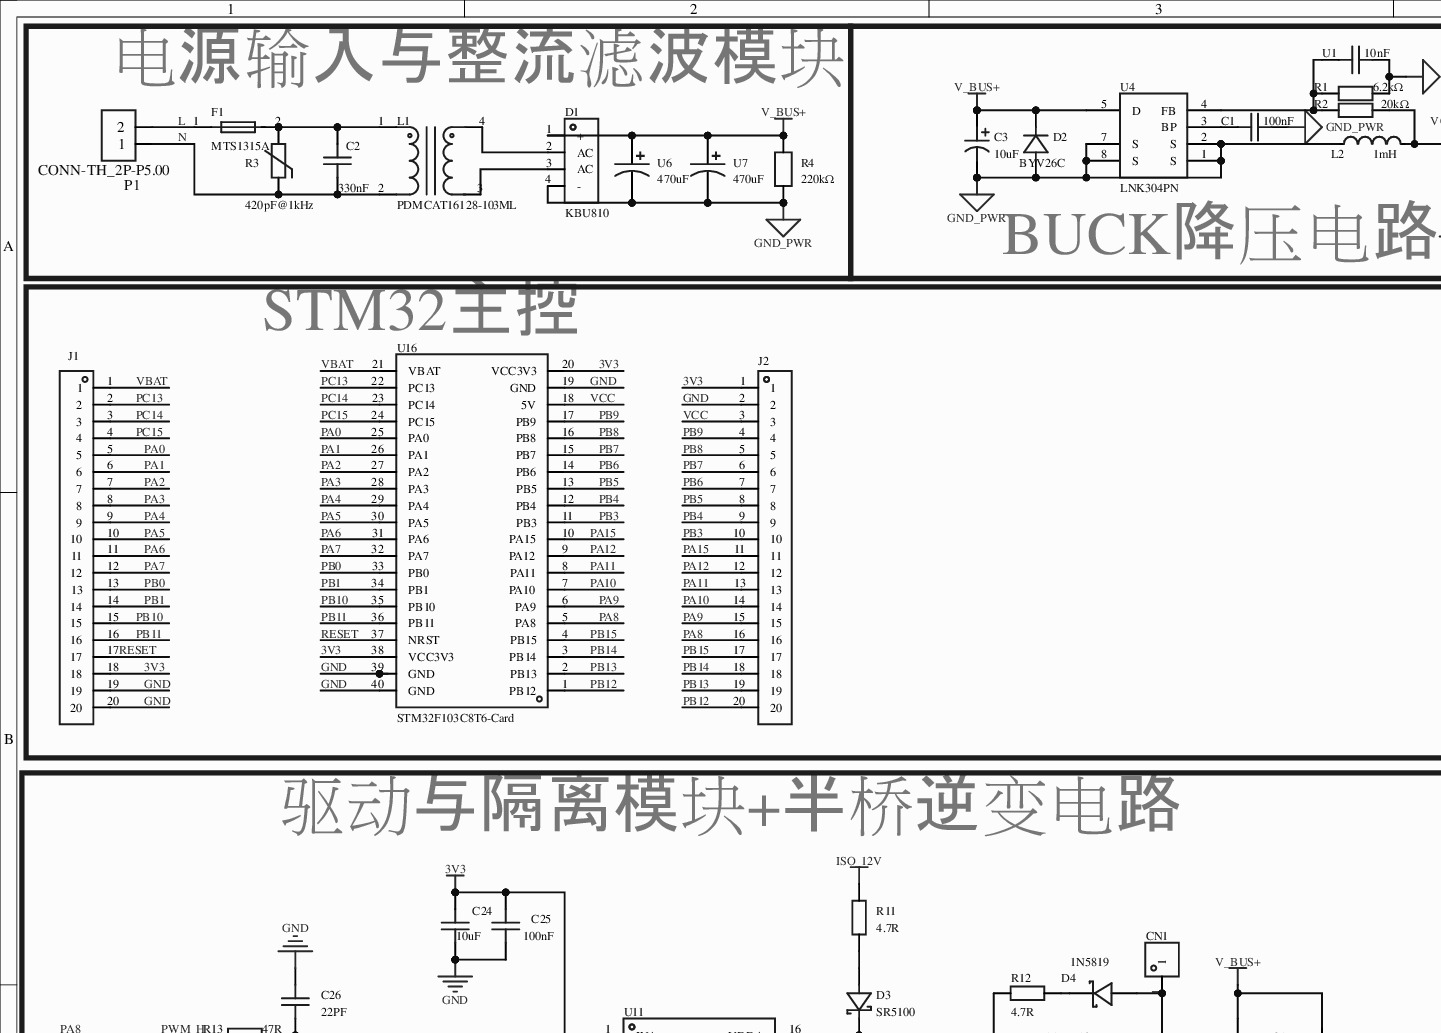
[diagram p0: MISC51807-3.schdoc, top left]
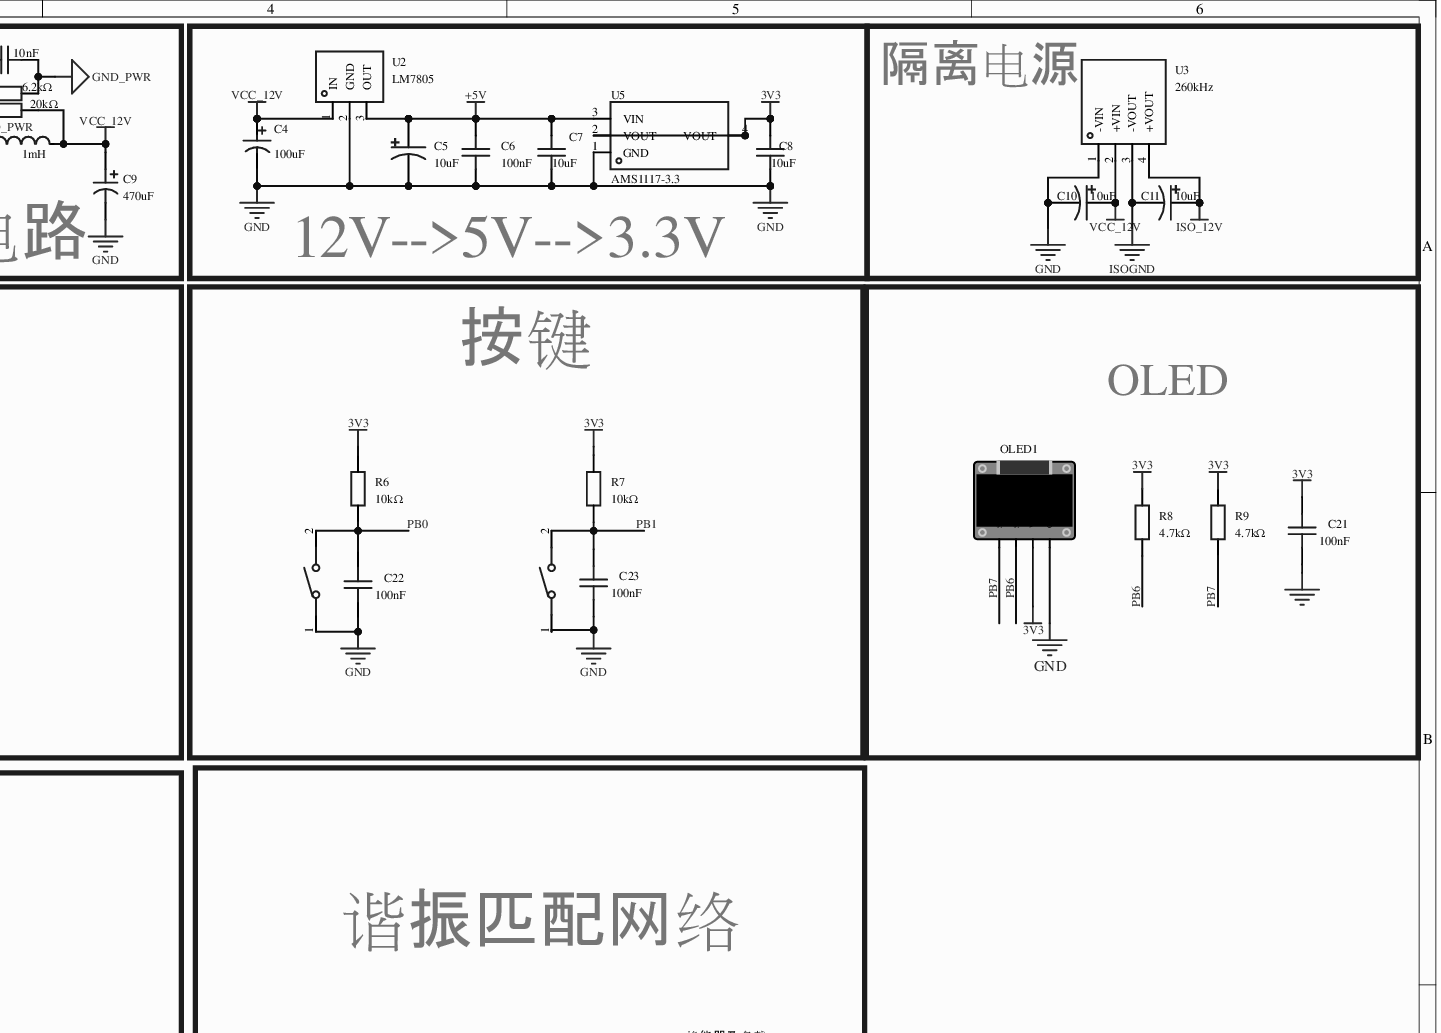
[diagram p1: MISC51807-3.schdoc, top right]
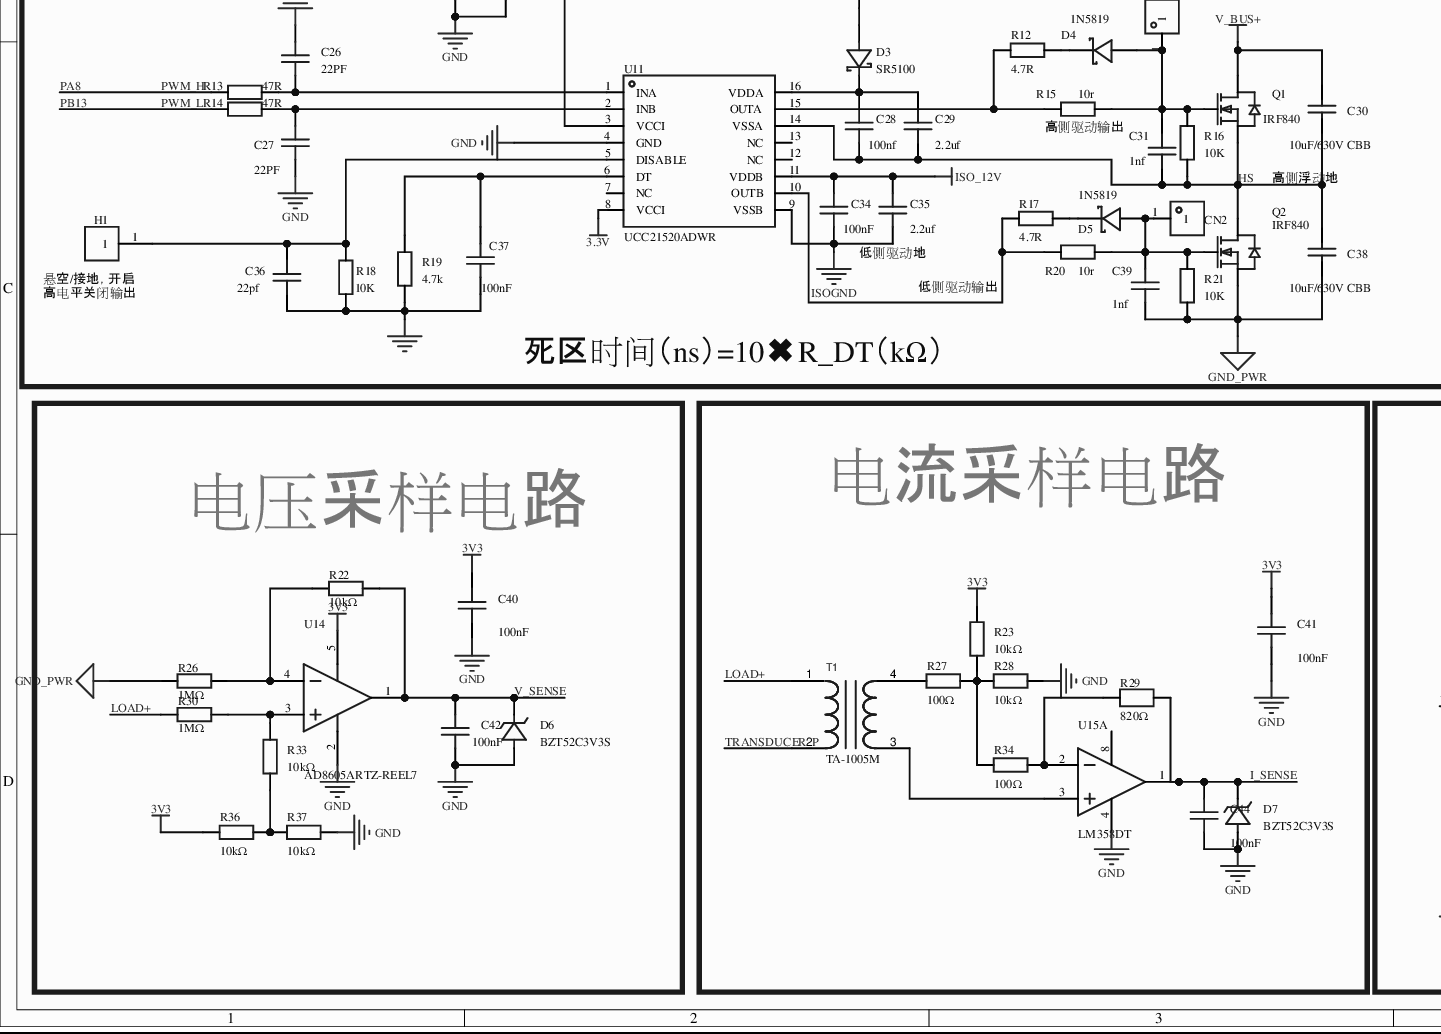
[diagram p2: MISC51807-3.schdoc, bottom left]
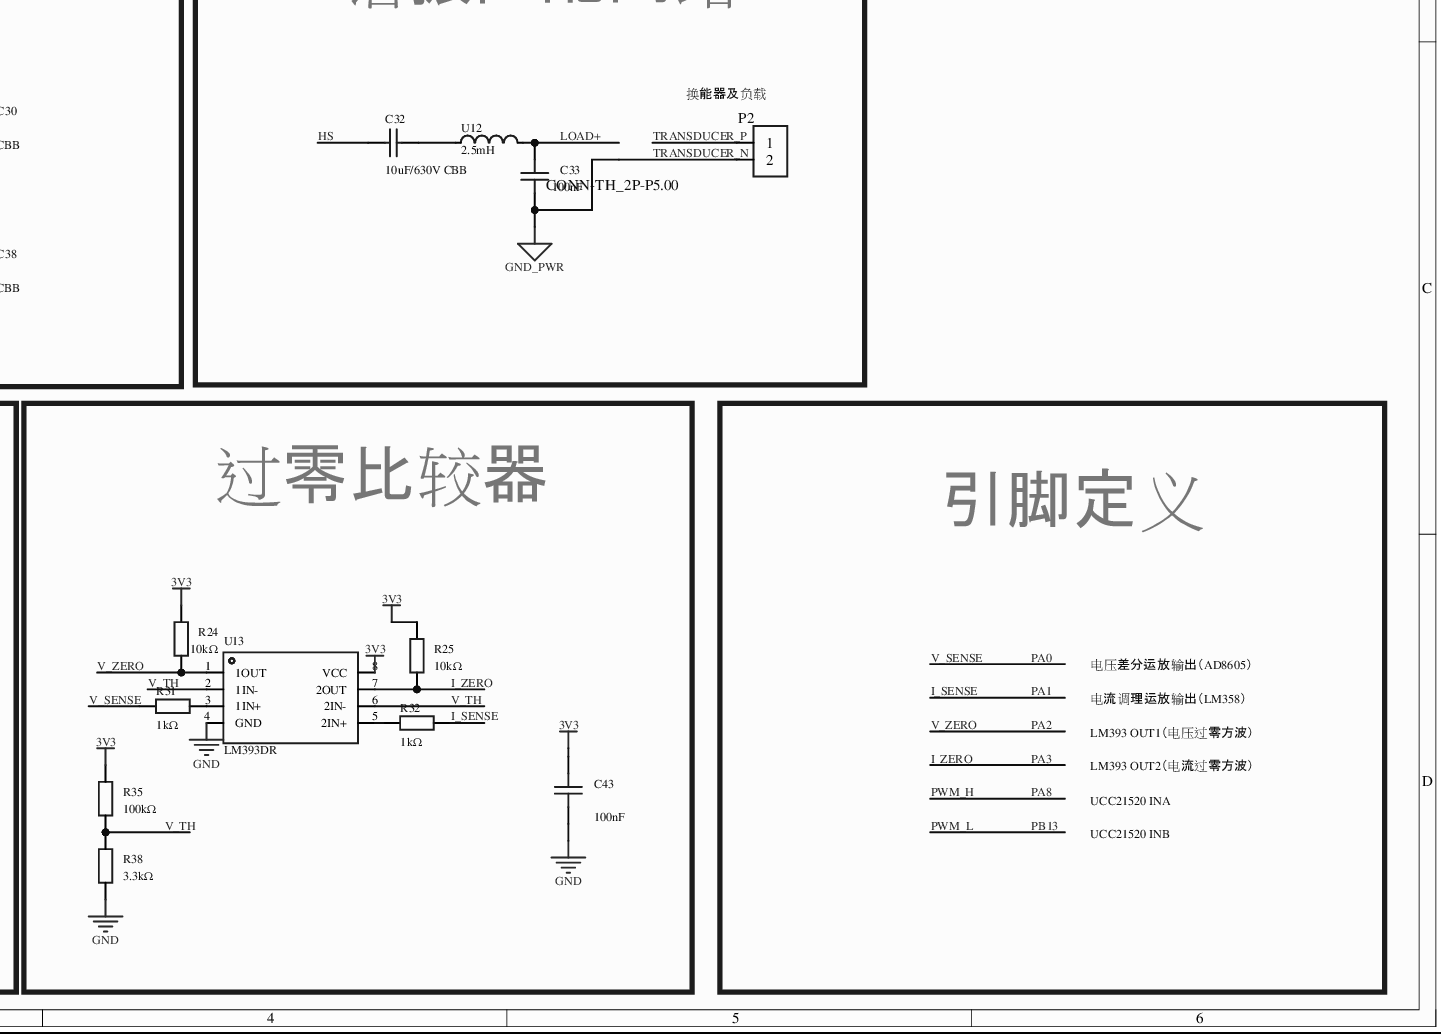
[diagram p3: MISC51807-3.schdoc, bottom right]
# Altium project MISC51807-2.PrjPcb (part 1 of 2)
1 sheet, 107 parts. Net scope: global (net labels, ports and power ports of the same name join across sheets).
Board file: MISC51807.pcbdoc

## Sheet MISC51807-3.schdoc
size 420 x 297 mm; Version: V1.0; @Project Name: MISC51807; @Update Date: 2026-04-01; @Create Date: 2026-04-01; @Board Name: MISC51807; @Create Time: 11:12:14; @Page Count: 1; @Page No: 1; @Schematic Name: MISC51807; @Update Time: 11:12:14; Size: A4

### Parts
C1  100nF  [CAP-TH_L5.0-W2.5-P5.00-D1.0]
C2  330nF  [CAP-TH_L18.0-W7.0-P15.00-D0.7]
C3  10uF  [CAP-TH_BD10.0-P5.00-D0.6-FD_1]
C4  100uF  [CAP-SMD_BD6.3-L6.6-W6.6-FD]
C5  10uF  [CAP-SMD_BD4.0-L4.3-W4.3-FD]
C6  100nF  [CAP-TH_L5.0-W2.5-P5.00-D1.0]
C7  10uF  [C0805]
C8  10uF  [C0805]
C9  470uF  [CAP-SMD_BD8.0-L8.3-W8.3-LS9.2-FD-H10.5]
C10  10uF  [CAP-SMD_BD4.0-L4.3-W4.3-FD_1]
C11  10uF  [CAP-SMD_BD4.0-L4.3-W4.3-FD_1]
C21  100nF  [C0603]
C22  100nF  [C0603]
C23  100nF  [C0603]
C24  10uF  [C0805]
C25  100nF  [C0603]
C26  22PF  [C0805]
C27  22PF  [C0805]
C28  100nf  [C0805]
C29  2.2uf  [C0805]
C30  10uF/630V CBB  [1uf/630V CBB]
C31  1nf  [C0805]
C32  10uF/630V CBB  [1uf/630V CBB]
C33  100nF  [C0603]
C34  100nF  [C0805]
C35  2.2uf  [C0805]
C36  22pf  [C0805]
C37  100nF  [C0805]
C38  10uF/630V CBB  [1uf/630V CBB]
C39  1nf  [C0805]
C40  100nF  [C0603]
C41  100nF  [C0603]
C42  100nF  [C0603]
C43  100nF  [C0603]
C44  100nF  [C0603]
CN1  RH-5001  [TEST-TH_BD2.54-P1.4_BLACK]  (value not drawn)
CN2  RH-5001  [TEST-TH_BD2.54-P1.4_BLACK]  (value not drawn)
D1  KBU810  [DIO-BG-TH_L23.2-W6.8-P5.10_KBU]
D2  BYV26C  [DO-41_BD2.6-L5.1-P9.00-D0.8-RD]
D3  SR5100  [DO-201AD_BD5.3-L8.4-P12.50-D1.4-RD]
D4  1N5819  [DO-41_BD2.4-L4.7-P8.70-D0.9-FD]
D5  1N5819  [DO-41_BD2.4-L4.7-P8.70-D0.9-FD]
D6  BZT52C3V3S  [SOD-323_L1.7-W1.3-LS2.6-RD]
D7  BZT52C3V3S  [SOD-323_L1.7-W1.3-LS2.6-RD]
F1  MTS1315A  [FUSE-TH_L8.4-W4.0-P5.08-D0.6]
H1  PZ254V-11-01P  [HDR-TH_1P-P2.54-V-M]  (value not drawn)
J1  2.54-1*20P直针  [HDR-TH_20P-P2.54-V-M-1]  (value not drawn)
J2  2.54-1*20P直针  [HDR-TH_20P-P2.54-V-M-1]  (value not drawn)
L1  PDMCAT16128-103ML  [IND-TH_4P-L20.0-W12.0-P6.00-LS10.0-BL]
L2  1mH  [IND-TH_BD8.5-P5.00-D0.6]
OLED1  (no value)  [0.96OLED_4P]
P1  CONN-TH_2P-P5.00  [CONN-TH_2P-P5.00]
P2  CONN-TH_2P-P5.00  [CONN-TH_2P-P5.00]
Q1  IRF840  [TO-220-3_L10.2-W4.5-P2.54-L-1]
Q2  IRF840  [TO-220-3_L10.2-W4.5-P2.54-L-1]
R1  6.2kΩ  [R0603]
R2  20kΩ  [R0603]
R3  420pF@1kHz  [RES-TH_L15.5-W5.6-P7.50-D0.8-S1.90]
R4  220kΩ  [RES-TH_BD3.9-L9.0-P13.00-D0.8]
R6  10kΩ  [R0603_1]
R7  10kΩ  [R0603_1]
R8  4.7kΩ  [R0603]
R9  4.7kΩ  [R0603]
R11  4.7R  [R0805]
R12  4.7R  [R0805]
R13  47R  [R0805]
R14  47R  [R0805]
R15  10r  [R0805]
R16  10K  [R0805]
R17  4.7R  [R0805]
R18  10K  [R0805]
R19  4.7k  [R0805]
R20  10r  [R0805]
R21  10K  [R0805]
R22  10kΩ  [R0805]
R23  10kΩ  [R0805]
R24  10kΩ  [R0805]
R25  10kΩ  [R0805]
R26  1MΩ  [R1206]
R27  100Ω  [R0805]
R28  10kΩ  [R0805]
R29  820Ω  [R0805]
R30  1MΩ  [R1206]
R31  1kΩ  [R0603]
R32  1kΩ  [R0603]
R33  10kΩ  [R0805]
R34  100Ω  [R0805]
R35  100kΩ  [R0603]
R36  10kΩ  [R0805]
R37  10kΩ  [R0805]
R38  3.3kΩ  [R0603_NEW]
SW2  TS-1088-AR02016  [SW-SMD_L3.9-W3.0-P4.45]  (value not drawn)
SW3  TS-1088-AR02016  [SW-SMD_L3.9-W3.0-P4.45]  (value not drawn)
T1  TA-1005M  [TA-1005M]
U1  10nF  [CAP-TH_L5.0-W2.5-P2.50-D0.5]
U2  LM7805  [TO-220-3_L10.0-W4.5-P2.54-L]
U3  260kHz  [PWRM-TH_4P-L11.5-W6.0-P2.54_B1503S]
U4  LNK304PN  [DIP-8_7P-L9.7-W6.4-P2.54-LS7.6-BL-PE6]
U5  AMS1117-3.3  [SOT-223-3_L6.5-W3.4-P2.30-LS7.0-BR]
U6  470uF  [CAP-TH_BD35.0-P10.00-D1.5-FD]
U7  470uF  [CAP-TH_BD35.0-P10.00-D1.5-FD]
U11  UCC21520ADWR  [SOIC-16_L10.3-W7.5-P1.27-LS10.3-BL]
U12  2.5mH  [IND-TH_BD9.5-P5.00-D0.7]
U13  LM393DR  [SOIC-8_L5.0-W4.0-P1.27-LS6.0-BL]
U14  AD8605ARTZ-REEL7  [SOT-23-5_L3.0-W1.7-P0.95-LS2.8-BR]
U15  LM358DT  [SOIC-8_L4.9-W3.9-P1.27-LS6.0-BL]  (part A of 2)
U16  STM32F103C8T6-Card  [CONN-TH_L53.3-W22.9_STM32F103C8T6-CARD]

### Blocks framed on the sheet
电源输入与整流滤波模块: C2 D1 F1 L1 P1 R3 R4 U6 U7
BUCK降压电路: C1 C3 C9 D2 L2 R1 R2 U1 U4
12V-->5V-->3.3V: C4-C8 U2 U5
隔离电源: C10 C11 U3
STM32主控: J1 J2 U16
按键: C22 C23 R6 R7 SW2 SW3
OLED: C21 OLED1 R8 R9
驱动与隔离模块+半桥逆变电路: C24-C31 C34-C39 CN1 CN2 D3-D5 H1 Q1 Q2 R11-R21 U11
谐振匹配网络: C32 C33 P2 U12
电压采样电路: C40 C42 D6 R22 R26 R30 R33 R36 R37 U14
电流采样电路: C41 C44 D7 R23 R27-R29 R34 T1 U15
过零比较器: C43 R24 R25 R31 R32 R35 R38 U13

### Nets
3.3V: U11.8(VCCI)
3V3: C8.2 C21.2 C24.2 C25.2 C40.1 C41.1 C43.1 J1.18 J2.1 OLED1.2(VCC) R6.2 R7.2 R8.2 R9.2 R23.1 R24.1 R25.1 R35.2 R36.2 U5.2(VOUT) U5.4(VOUT) U11.3(VCCI) U13.8(VCC) U14.5(+V) U16.20(VCC3V3) U16.38(VCC3V3)
+5V: C5.1 C6.2 C7.2 U2.3(OUT) U5.3(VIN)
GND: C4.2 C5.2 C6.1 C7.1 C8.1 C9.2 C10.2 C21.1 C22.1 C23.1 C24.1 C25.1 C26.2 C27.1 C36.1 C37.1 C40.2 C41.2 C42.1 C43.2 C44.2 D6.2(A) D7.2(A) J1.19 J1.20 J2.2 OLED1.1(GND) R18.1 R19.1 R28.2 R37.1 R38.1 SW2.1 SW3.1 U2.2(GND) U3.1(-VIN) U5.1(GND) U11.4(GND) U13.4(GND) U14.2(-V) U15.4(VCC-/GND) U16.19(GND) U16.39(GND) U16.40(GND)
ISO_12V: C11.1 C34.1 C35.1 R11.1 U3.4(+VOUT) U11.11(VDDB)
ISOGND: C11.2 C34.2 C35.2 U3.3(-VOUT) U11.9(VSSB)
GND_PWR: C1.1 C3.2 C33.1 C38.2 C39.1 D1.4(-) D2.2(A) L2.1 P2.2 Q2.3(S) R1.1 R4.1 R21.1 R26.1 U1.1 U4.1(S) U4.2(S) U4.7(S) U4.8(S) U6.2 U7.2  [also labelled TRANSDUCER_N]
V_BUS+: C3.1 C30.1 D1.1(+) D2.1(K) Q1.2(D) R4.2 U4.5(D) U6.1 U7.1
VCC_12V: C4.1 C9.1 C10.1 L2.2 R2.1 U2.1(IN) U3.2(+VIN)
HS: C28.2 C29.2 C30.2 C31.1 C32.1 C38.1 Q1.3(S) Q2.2(D) R16.1 U11.14(VSSA)
I_SENSE: C44.1 D7.1(K) J1.6 R29.1 R32.2 U15.1(OUT1) U16.26(PA1)  [also labelled PA1]
I_ZERO: J1.8 R25.2 U13.7(2OUT) U16.28(PA3)  [also labelled PA3]
L: F1.1 P1.2
LOAD+: C33.2 R30.1 T1.1 U12.2
N: C2.1 L1.2 P1.1 R3.1
PA0: C42.2 D6.1(K) J1.5 R22.2 R31.1 U14.1(OUT) U16.25(PA0)  [also labelled V_SENSE]
PA2: J1.7 R24.2 U13.1(1OUT) U16.27(PA2)  [also labelled V_ZERO]
PA4: J1.9 U16.29(PA4)
PA5: J1.10 U16.30(PA5)
PA6: J1.11 U16.31(PA6)
PA7: J1.12 U16.32(PA7)
PA8: J2.16 R13.1 U16.5(PA8)  [also labelled PWM_H]
PA9: J2.15 U16.6(PA9)
PA10: J2.14 U16.7(PA10)
PA11: J2.13 U16.8(PA11)
PA12: J2.12 U16.9(PA12)
PA15: J2.11 U16.10(PA15)
PB0: C22.2 J1.13 R6.1 SW2.2 U16.33(PB0)
PB1: C23.2 J1.14 R7.1 SW3.2 U16.34(PB1)
PB3: J2.10 U16.11(PB3)
PB4: J2.9 U16.12(PB4)
PB5: J2.8 U16.13(PB5)
PB6: J2.7 OLED1.3(SCL) R8.1 U16.14(PB6)
PB7: J2.6 OLED1.4(SDA) R9.1 U16.15(PB7)
PB8: J2.5 U16.16(PB8)
PB9: J2.4 U16.17(PB9)
PB10: J1.15 U16.35(PB10)
PB11: J1.16 U16.36(PB11)
PB12: J2.20 U16.1(PB12)
PB13: J2.19 R14.1 U16.2(PB13)  [also labelled PWM_L]
PB14: J2.18 U16.3(PB14)
PB15: J2.17 U16.4(PB15)
PC13: J1.2 U16.22(PC13)
PC14: J1.3 U16.23(PC14)
PC15: J1.4 U16.24(PC15)
RESET: J1.17 U16.37(NRST)
TRANSDUCER_P: P2.1 T1.2
V_TH: R35.1 R38.2 U13.2(1IN-) U13.6(2IN-)
VBAT: J1.1 U16.21(VBAT)
VCC: J2.3 U16.18(5V)
NetC1_2: C1.2 U4.3(BP)
NetC2_2: C2.2 F1.2 L1.1 R3.2
NetC26_1: C26.1 R13.2 U11.1(INA)
NetC27_2: C27.2 R14.2 U11.2(INB)
NetC28_1: C28.1 C29.1 D3.1 U11.16(VDDA)
NetC31_2: C31.2 CN1.1 D4.1(A) Q1.1(G) R15.1 R16.2
NetC32_2: C32.2 U12.1
NetC36_2: C36.2 H1.1 R18.2 U11.5(DISABLE)
NetC37_2: C37.2 R19.2 U11.6(DT)
NetC39_2: C39.2 CN2.1 D5.1(A) Q2.1(G) R20.1 R21.2
NetD1_2: D1.2(AC) L1.4
NetD1_3: D1.3(AC) L1.3
NetD3_2: D3.2 R11.2
NetD4_2: D4.2(K) R12.2
NetD5_2: D5.2(K) R17.2
NetR1_2: R1.2 R2.2 U1.2 U4.4(FB)
NetR12_1: R12.1 R15.2 U11.15(OUTA)
NetR17_1: R17.1 R20.2 U11.10(OUTB)
NetR22_1: R22.1 R26.2 U14.4(-IN)
NetR23_2: R23.2 R27.2 R28.1 R34.2
NetR27_1: R27.1 T1.4
NetR29_2: R29.2 R34.1 U15.2(IN1-)
NetR30_2: R30.2 R33.2 U14.3(+IN)
NetR31_2: R31.2 U13.3(1IN+)
NetR32_1: R32.1 U13.5(2IN+)
NetR33_1: R33.1 R36.1 R37.2
NetT1_3: T1.3 U15.3(IN1+)

Not connected (* = marked no-connect by the designer): U11 7(NC)* 12(NC)* 13(NC)*; U15 8(VCC+)

### Notes on the sheet
- (near R15) 高侧驱动输出
- (near P2) 换能器及负载
- 高侧浮动地
- (near H1) 悬空/接地，开启
  高电平关闭输出
- 低侧驱动地
- 低侧驱动输出
- 死区时间（ns）=10✖R_DT（kΩ）
- 引脚定义
- 电压差分运放输出（AD8605）
- 电流调理运放输出（LM358）
- LM393 OUT1（电压过零方波）
- LM393 OUT2（电流过零方波）
- UCC21520 INA
- UCC21520 INB

### Library data of the parts
C1 C6 = CC1H104MC1FD3F6C10MF: 容值:100nF;精度:±20%;额定电压:50V;温度系数:Y5V;; Manufacturer: Dersonic(德尔创); AddInBom: yes; ModelId: 08e3d7481fc7486bb1b263873f51e1e10819f05c4eef4c71ace90d822a990e87; ModelName: CAP-TH_BD5.0-W2.5-P5.08; ModelTransform: 224.652,98.425,0,0,0,0,-0.005,0,-137.795; Tolerance: ±20%; Voltage Rating: 50V; Pin Spacing: 5.08mm; Temperature Coefficient: Y5V; Body Thickness: 2.2mm; Symbol: CC1H104MC1FD3F6C10MF; Device: CC1H104MC1FD3F6C10MF; LCSC Part Name: 100nF ±20% 50V; SupplierPart: C254085; ManufacturerPart: CC1H104MC1FD3F6C10MF; Supplier Footprint: 插件,P=5.08mm; JLCPCB Part Class: Extended Part; Datasheet: https://item.szlcsc.com/datasheet/CC1H104MC1FD3F6C10MF/248635.html; Supplier: LCSC; ConvertToPcb: yes; FootprintName: CAP-TH_L5.0-W2.5-P5.00-D1.0; Value: 100nF; Diameter: 6mm
C2 = MKP62-275VAC/334: 容值:330nF;精度:±10%;额定电压:275V;; Manufacturer: 东通电子; AddInBom: yes; ModelId: 9627c4034b1444ca8cb0a2a63be374ac0819f05c4eef4c71ace90d822a990e87; ModelTransform: 708.66,275.59,0,0,0,0,0,0,-196.85; Tolerance: ±10%; Voltage Rating: 275V; Symbol: MKP62-275VAC/334; Device: MKP62-275VAC/334; LCSC Part Name: 330nF ±10% 275V; SupplierPart: C2913191; ManufacturerPart: MKP62-275VAC/334; Supplier Footprint: 插件,P=15mm; JLCPCB Part Class: Extended Part; Datasheet: https://item.szlcsc.com/datasheet/MKP62-275VAC%252F334/3198288.html; Supplier: LCSC; ConvertToPcb: yes; FootprintName: CAP-TH_L18.0-W7.0-P15.00-D0.7; ModelName: CAP-TH_L18.0-W7.0-P15.00-D0.7; Value: 330nF
C3 = ERG450V10M10x16: 容值:10uF;精度:±20%;额定电压:450V;纹波电流:100mA@100kHz;等效串联电阻(ESR):9.45Ω@100kHz;; Manufacturer: JIERR(捷而瑞); AddInBom: yes; ModelId: c24ffaad515542988ee7b6ee8c6416550819f05c4eef4c71ace90d822a990e87; ModelName: CAP-TH_BD10.0-P5.00-D0.6-FD-H12.5; ModelTransform: 394.094,393.57658,0,0,0,0,0,0,-137.795; Tolerance: ±20%; Voltage Rating: 450V; Pin Spacing: 5mm; Lifetime: 2000hrs@105℃; Symbol: ERG450V10M10X16; Device: ERG450V10M10x16; LCSC Part Name: 10uF ±20% 450V; SupplierPart: C46552835; ManufacturerPart: ERG450V10M10x16; Supplier Footprint: 插件,D10xL16mm; JLCPCB Part Class: Extended Part; Datasheet: https://item.szlcsc.com/datasheet/ERG450V10M10x16/48687203.html; Supplier: LCSC; ConvertToPcb: yes; FootprintName: CAP-TH_BD10.0-P5.00-D0.6-FD_1; Value: 10uF; Ripple Current: 100mA@100kHz; Equivalent Series Resistance(ESR): 9.45Ω@100kHz; Diameter: 10mm; Height - Seated (Max): 16mm; Operating Temperature: -25℃~+105℃
C4 = RVT1E101M0607_C72477: 容值:100uF;精度:±20%;额定电压:25V;纹波电流:93mA@120Hz;等效串联电阻(ESR):-;; Manufacturer: ROQANG(容强); Symbol: RVT1E101M0607-C72477; AddInBom: yes; ModelId: ec7f1c7bda5e4386b54ec5ff3d1d94ff0819f05c4eef4c71ace90d822a990e87; ModelTransform: 307.086,259.842,0,180,0,0,0,0,0; Tolerance: ±20%; Voltage Rating: 25V; Lifetime: 2000hrs@105℃; Device: RVT1E101M0607_C72477; LCSC Part Name: 100uF ±20% 25V; SupplierPart: C72477; ManufacturerPart: RVT1E101M0607; Supplier Footprint: SMD,D6.3xL7.7mm; JLCPCB Part Class: Extended Part; Datasheet: https://item.szlcsc.com/datasheet/RVT1E101M0607/73588.html; Supplier: LCSC; ConvertToPcb: yes; FootprintName: CAP-SMD_BD6.3-L6.6-W6.6-FD; ModelName: CAP-SMD_BD6.3-L6.6-W6.6-FD; Value: 100uF; Ripple Current: 93mA@120Hz; Equivalent Series Resistance(ESR): -; Diameter: 6.3mm; Height - Seated (Max): 7.7mm; Operating Temperature: -40℃~+105℃
C5 = VT1C100M0405: 容值:10uF;精度:±20%;额定电压:16V;纹波电流:17mA@120Hz;等效串联电阻(ESR):-;; Manufacturer: ROQANG(容强); AddInBom: yes; ModelId: d5abac2407cc4bb7a22453350802a0e20819f05c4eef4c71ace90d822a990e87; ModelName: CAP-SMD_L4.3-W4.3-H5.3-LS5.1; ModelTransform: 169.291,181.102,0,90,0,0,0.376,-0.001,0; Tolerance: ±20%; Voltage Rating: 16V; Lifetime: 2000hrs@105℃; Symbol: VT1C100M0405; Device: VT1C100M0405; LCSC Part Name: 10uF ±20% 16V; SupplierPart: C213487; ManufacturerPart: VT1C100M0405; Supplier Footprint: SMD,D4xL5.4mm; JLCPCB Part Class: Extended Part; Supplier: LCSC; ConvertToPcb: yes; FootprintName: CAP-SMD_BD4.0-L4.3-W4.3-FD; Value: 10uF; Ripple Current: 17mA@120Hz; Equivalent Series Resistance(ESR): -; Diameter: 4mm; Height - Seated (Max): 5.4mm; Operating Temperature: -40℃~+105℃
C7 C8 C24 = C0805X106K010T: 容值:10uF;精度:±10%;额定电压:10V;温度系数:X7R;; Manufacturer: IHHEC(禾伸堂); AddInBom: yes; ModelId: 1ba041120af144c991958decab20d2410819f05c4eef4c71ace90d822a990e87; ModelName: C0805_L2.0-W1.3-H1.3; ModelTransform: 78.74,51.181,0,0,0,0,0,0.0005,0; Tolerance: ±10%; Voltage Rating: 10V; Temperature Coefficient: X7R; Symbol: C0805X106K010T; Device: C0805X106K010T; LCSC Part Name: 10uF ±10% 10V; SupplierPart: C340314; ManufacturerPart: C0805X106K010T; Supplier Footprint: 0805; JLCPCB Part Class: Extended Part; Datasheet: https://item.szlcsc.com/datasheet/C0805X106K010T/317654.html; Supplier: LCSC; ConvertToPcb: yes; FootprintName: C0805; Value: 10uF
C9 = RV35V470M8X10: 容值:470uF;精度:±20%;额定电压:35V;; Manufacturer: JIERR(捷而瑞); AddInBom: yes; Tolerance: ±20%; Voltage Rating: 35V; Lifetime: 5000hrs@105℃; ModelId: 972af18cf9b34067b21b9c7338aea287; Symbol: RV35V470M8X10; Device: RV35V470M8X10; LCSC Part Name: 470uF ±20% 35V; SupplierPart: C48935389; ManufacturerPart: RV35V470M8X10; Supplier Footprint: SMD,D8xL10.5mm; JLCPCB Part Class: Extended Part; Datasheet: https://item.szlcsc.com/datasheet/RV35V470M8X10/51248509.html; Supplier: LCSC; ConvertToPcb: yes; FootprintName: CAP-SMD_BD8.0-L8.3-W8.3-LS9.2-FD-H10.5; Value: 470uF; Diameter: 8mm; Height - Seated (Max): 10.5mm; Operating Temperature: -55℃~+105℃; ModelName: CAP-SMD_BD8.0-L8.3-W8.3-LS9.2-FD-H10.5
C10 C11 = VT1E100M0405: 容值:10uF;精度:±20%;额定电压:25V;纹波电流:15mA@120Hz;等效串联电阻(ESR):-;; Manufacturer: ROQANG(容强); AddInBom: yes; ModelId: d5abac2407cc4bb7a22453350802a0e20819f05c4eef4c71ace90d822a990e87; ModelName: CAP-SMD_L4.3-W4.3-H5.3-LS5.1; ModelTransform: 169.291,181.102,0,90,0,0,0,-0.593,0; Tolerance: ±20%; Voltage Rating: 25V; Lifetime: 2000hrs@105℃; Symbol: VT1E100M0405; Device: VT1E100M0405; LCSC Part Name: 10uF ±20% 25V; SupplierPart: C213486; ManufacturerPart: VT1E100M0405; Supplier Footprint: SMD,D4xL5.4mm; JLCPCB Part Class: Extended Part; Supplier: LCSC; ConvertToPcb: yes; FootprintName: CAP-SMD_BD4.0-L4.3-W4.3-FD_1; Value: 10uF; Ripple Current: 15mA@120Hz; Equivalent Series Resistance(ESR): -; Diameter: 4mm; Height - Seated (Max): 5.4mm; Operating Temperature: -40℃~+105℃
C21-C23 C25 C33 C40-C44 = CC0603KRX7R9BB104_1: 容值:100nF;精度:±10%;额定电压:50V;材质(温度系数):X7R;; Manufacturer: YAGEO(国巨); 3D Model: ac125912035d415993ca9572d50418b1; 3D Model Transform: 62.992,31.496,0,0,0,0,0,0,0; Tolerance: ±10%; Voltage Rated: 50V; Temperature Coefficient: X7R; AddInBom: yes; ModelName: C0603_L1.6-W0.8-H0.8; Symbol: CC0603KRX7R9BB104_1; Device: CC0603KRX7R9BB104_1; Value: 100nF; LCSC Part Name: 100nF ±10% 50V; Supplier Part: C14663; Manufacturer Part: CC0603KRX7R9BB104; Supplier Footprint: 0603; JLCPCB Part Class: Basic Part; Datasheet: https://atta.szlcsc.com/upload/public/pdf/source/20170116/1484561234239.pdf; Supplier: LCSC; ConvertToPcb: yes; FootprintName: C0603
C26 C27 = CAP_0805: Symbol: CapAcitance; 3D Model: 1ba041120af144c991958decab20d241; 3D Model Transform: 78.74,51.181,0,0,0,0,0,0.0005,0; Value: 100nF; ConvertToPcb: yes; ModelName: C0805_L2.0-W1.3-H1.3; Device: CAP_0805; Supplier Footprint: 0805; AddInBom: yes; FootprintName: C0805
C28 C29 C31 C34-C37 C39 = CAP_0805: Symbol: CapAcitance; 3D Model: 1ba041120af144c991958decab20d241; 3D Model Transform: 78.74,51.181,0,0,0,0,0,0.0005,0; ConvertToPcb: yes; ModelName: C0805_L2.0-W1.3-H1.3; Device: CAP_0805; Supplier Footprint: 0805; AddInBom: yes; FootprintName: C0805
  C28: Value: 100nf
  C29 C35: Value: 2.2uf
  C31 C39: Value: 1nf
  C34 C37: Value: 100nF
  C36: Value: 22pf
C30 C32 C38 = 1uF/630V CBB: Symbol: Cap; AddInBom: yes; Device: 1uF/630V CBB; Published: 8-Jun-2000; LatestRevisionDate: 17-Jul-2002; LatestRevisionNote: Re-released for DXP Platform.; PackageReference: RAD-0.3; PackageDescription: Radial Cap, Thru-Hole; 2 Leads; 0.3 in Pin Spacing; ConvertToPcb: yes; FootprintName: 1uf/630V CBB; Publisher: Altium Limited
CN1 CN2 = RH-5001: 测试针  高温尼龙/磷青铜镀银 5001测试点 100x80mm; Manufacturer: 荣和; 3D Model: 3b56df8954204a2c9a7df7bc4a4fe082; 3D Model Transform: 98.425,98.79098,0,0,0,0,0,0,-137.795; Connector Type: 插针型(穿板); Plastic Color: 黑色; Board Space (Diameter φ/ Length x Width): 2.5mm; AddInBom: yes; Symbol: RH-5001; Device: RH-5001; LCSC Part Name: PCB电路板测试点/测试针; Supplier Part: C5199801; Manufacturer Part: RH-5001; Supplier Footprint: -; JLCPCB Part Class: 扩展库; Datasheet: https://atta.szlcsc.com/upload/public/pdf/source/20240125/4C7D900D13ECC10386B63F24462DBAAB.pdf; Supplier: LCSC; ConvertToPcb: yes; FootprintName: TEST-TH_BD2.54-P1.4_BLACK; ModelName: TEST-TH_BD2.54-P1.4_BLACK
D1 = KBU810_C34835: 正向压降(Vf):1.1V@8A;直流反向耐压(Vr):1kV;整流电流:8A;非重复峰值浪涌电流 (Ifsm):300A;; Manufacturer: MDD(辰达半导体); AddInBom: yes; ModelId: 7c798be3ead04ff187532d242bb1ef440819f05c4eef4c71ace90d822a990e87; ModelName: DIO-BG-TH_KBU-L23.2-W6.8-H19.2-P5.10; ModelTransform: 905.51,259.842,0,0,0,0,-0.001,51.181,-137.795; Voltage - DC Reverse(Vr): 1kV; Current - Rectified: 8A; Reverse Leakage Current (Ir): 10uA@1kV; Non-Repetitive Peak Forward Surge Current: 300A; Operating Junction Temperature Range: -55℃~+150℃; Symbol: KBU810; Device: KBU810_C34835; LCSC Part Name: KBU810; SupplierPart: C34835; ManufacturerPart: KBU810; Supplier Footprint: KBU; JLCPCB Part Class: Extended Part; Datasheet: https://item.szlcsc.com/datasheet/KBU810/35805.html; Supplier: LCSC; ConvertToPcb: yes; FootprintName: DIO-BG-TH_L23.2-W6.8-P5.10_KBU; Voltage - Forward(Vf@If): 1.1V@8A